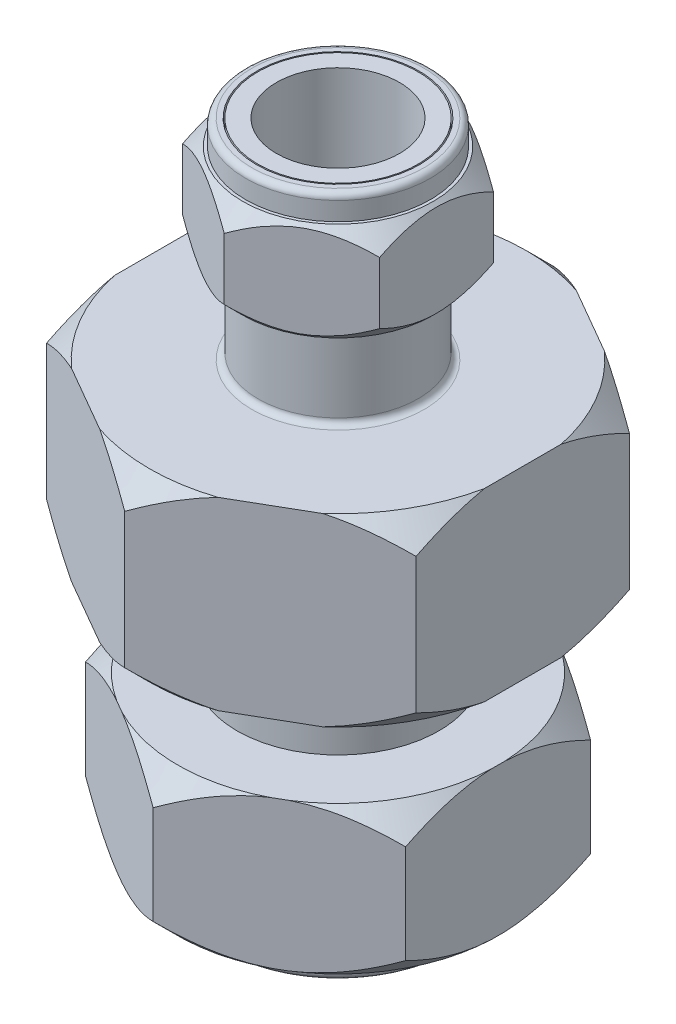
from build123d import *

# Parameters (mm, degrees)
BOSS_EXTRUDE1_DEPTH = 15
SKETCH2_R           = 6.5
BOSS_EXTRUDE2_DEPTH = 17
SKETCH3_R           = 8
BOSS_EXTRUDE3_DEPTH = 22
SKETCH4_R           = 6.5
CUT_EXTRUDE1_DEPTH  = 20
SKETCH5_R           = 5
CUT_EXTRUDE2_DEPTH  = 59.660037504
SKETCH6_R           = 7.5
SKETCH6_R_2         = 6.6
BOSS_EXTRUDE4_DEPTH = 2
SKETCH7_R           = 6.6
BOSS_EXTRUDE5_DEPTH = 8
SKETCH11_R          = 9.5
SKETCH11_R_2        = 8.2
BOSS_EXTRUDE6_DEPTH = 3
SKETCH12_R          = 8.2
BOSS_EXTRUDE7_DEPTH = 12
FILLET1_R           = 0.5
FILLET2_R           = 0.5
FILLET3_R           = 0.5


with BuildPart() as part:
    # Sketch1 → Boss-Extrude1 (new body)
    with BuildSketch(Plane(origin=(0, 0, 0), x_dir=(1, 0, 0), z_dir=(0, 1, 0))):
        Polygon((0, -17.320508076), (15, -8.660254038), (15, 8.660254038), (0, 17.320508076), (-15, 8.660254038), (-15, -8.660254038), align=None)
    extrude(amount=BOSS_EXTRUDE1_DEPTH)

    # Sketch2 → Boss-Extrude2 (add)
    with BuildSketch(Plane(origin=(0, 15, 0), x_dir=(1, 0, 0), z_dir=(0, 1, 0))):
        with Locations(Location((0, 0, 0), (0, 0, 270))):
            Circle(SKETCH2_R)
    extrude(amount=BOSS_EXTRUDE2_DEPTH)

    # Sketch3 → Boss-Extrude3 (add)
    with BuildSketch(Plane.XZ):
        with Locations(Location((0, 0, 0), (0, 0, 270))):
            Circle(SKETCH3_R)
    extrude(amount=BOSS_EXTRUDE3_DEPTH)

    # Sketch4 → Cut-Extrude1 (cut)
    with BuildSketch(Plane.XZ.offset(22)):
        with Locations(Location((0, 0, 0), (0, 0, 90))):
            Circle(SKETCH4_R)
    extrude(amount=-CUT_EXTRUDE1_DEPTH, mode=Mode.SUBTRACT)

    # Sketch5 → Cut-Extrude2 (cut, through all)
    with BuildSketch(Plane(origin=(0, 32, 0), x_dir=(1, 0, 0), z_dir=(0, 1, 0))):
        with Locations(Location((0, 0, 0), (0, 0, 270))):
            Circle(SKETCH5_R)
    extrude(amount=-CUT_EXTRUDE2_DEPTH, mode=Mode.SUBTRACT)


with BuildPart() as body_2:
    # Sketch6 → Boss-Extrude4 (new body)
    with BuildSketch(Plane(origin=(0, 32, 0), x_dir=(1, 0, 0), z_dir=(0, 1, 0))):
        with Locations(Location((0, 0, 0), (0, 0, 270))):
            Circle(SKETCH6_R)
        with Locations(Location((0, 0, 0), (0, 0, 270))):
            Circle(SKETCH6_R_2, mode=Mode.SUBTRACT)
    extrude(amount=-BOSS_EXTRUDE4_DEPTH)

    # Sketch7 → Boss-Extrude5 (add)
    with BuildSketch(Plane.XZ.offset(-30)):
        Polygon((0, 9.237604307), (-8, 4.618802154), (-8, -4.618802154), (0, -9.237604307), (8, -4.618802154), (8, 4.618802154), align=None)
        with Locations(Location((0, 0, 0), (0, 0, 90))):
            Circle(SKETCH7_R, mode=Mode.SUBTRACT)
    extrude(amount=BOSS_EXTRUDE5_DEPTH)


with BuildPart() as body_3:
    # Sketch11 → Boss-Extrude6 (new body)
    with BuildSketch(Plane.XZ.offset(22)):
        with Locations(Location((0, 0, 0), (0, 0, 270))):
            Circle(SKETCH11_R)
        with Locations(Location((0, 0, 0), (0, 0, 270))):
            Circle(SKETCH11_R_2, mode=Mode.SUBTRACT)
    extrude(amount=-BOSS_EXTRUDE6_DEPTH)

    # Sketch12 → Boss-Extrude7 (add)
    with BuildSketch(Plane(origin=(0, -19, 0), x_dir=(1, 0, 0), z_dir=(0, 1, 0))):
        Polygon((0, 15.011106999), (-13, 7.505553499), (-13, -7.505553499), (0, -15.011106999), (13, -7.505553499), (13, 7.505553499), align=None)
        with Locations(Location((0, 0, 0), (0, 0, 90))):
            Circle(SKETCH12_R, mode=Mode.SUBTRACT)
    extrude(amount=BOSS_EXTRUDE7_DEPTH)


with BuildPart() as cut_revolve2_tool:
    # Sketch9 → Cut-Revolve2 (revolve)
    with BuildSketch(Plane(origin=(0, 0, 0), x_dir=(0, 0, -1), z_dir=(1, 0, 0))):
        Polygon((-7.737604307, 30), (-9.237604307, 28.5), (-9.237604307, 30), align=None)
        Polygon((-9.237604307, 22), (-7.737604307, 22), (-9.237604307, 23.5), align=None)
        Polygon((-17.320508076, 15), (-17.320508076, 13), (-15.320508076, 15), align=None)
        Polygon((-15.320508076, 0), (-17.320508076, 0), (-17.320508076, 2), align=None)
        Polygon((-15.011106999, -7), (-15.011106999, -9), (-13.011106999, -7), align=None)
        Polygon((-13.011106999, -19), (-15.011106999, -19), (-15.011106999, -17), align=None)
    revolve(axis=Axis((0, 32, 0), (0, 1, 0)))


with BuildPart() as part_1:
    add(part.part)

    # Cut-Revolve2: cut by cut_revolve2_tool
    add(cut_revolve2_tool.part, mode=Mode.SUBTRACT)

    # Fillet2
    fillet2_edges = [part_1.edges().sort_by_distance(p)[0] for p in [
        (0, 15, -6.5),
        (0, 0, 8),
    ]]
    fillet(fillet2_edges, radius=FILLET2_R)


with BuildPart() as body_2_1:
    add(body_2.part)

    # Cut-Revolve2: cut by cut_revolve2_tool
    add(cut_revolve2_tool.part, mode=Mode.SUBTRACT)

    # Fillet1
    fillet1_edges = [body_2_1.edges().sort_by_distance(p)[0] for p in [
        (0, 32, -7.5),
    ]]
    fillet(fillet1_edges, radius=FILLET1_R)


with BuildPart() as body_3_1:
    add(body_3.part)

    # Cut-Revolve2: cut by cut_revolve2_tool
    add(cut_revolve2_tool.part, mode=Mode.SUBTRACT)

    # Fillet3
    fillet3_edges = [body_3_1.edges().sort_by_distance(p)[0] for p in [
        (0, -22, 9.5),
    ]]
    fillet(fillet3_edges, radius=FILLET3_R)


solid = Compound([part_1.part, body_2_1.part, body_3_1.part])
